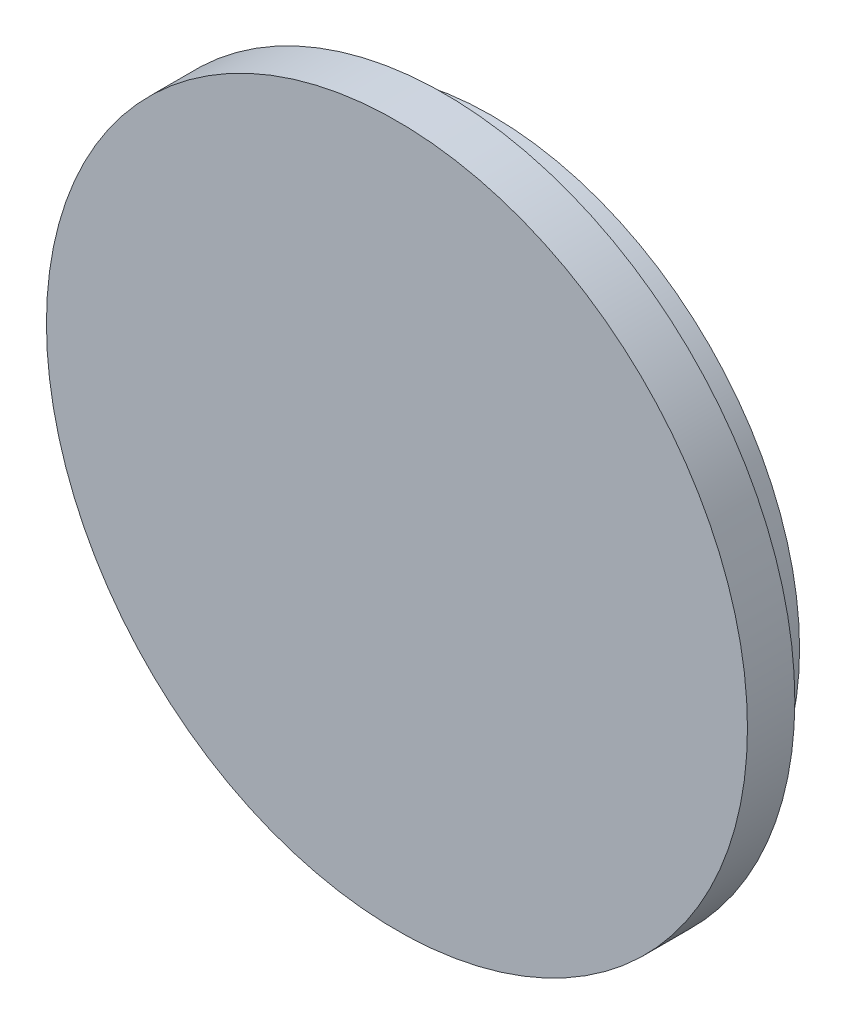
from build123d import *

# Parameters (mm, degrees)
SKETCH_1_R      = 7.4
EXTRUDE_1_DEPTH = 1
SKETCH_1_3_R    = 6.5
EXTRUDE_2_DEPTH = 1


with BuildPart() as part:
    # 草图1 → 凸台-拉伸1 (new body)
    with BuildSketch(Plane.XY):
        Circle(SKETCH_1_R)
    extrude(amount=EXTRUDE_1_DEPTH)

    # 草图1<3> → 凸台-拉伸2 (add)
    with BuildSketch(Plane.XY):
        Circle(SKETCH_1_3_R)
    extrude(amount=-EXTRUDE_2_DEPTH)


solid = part.part
